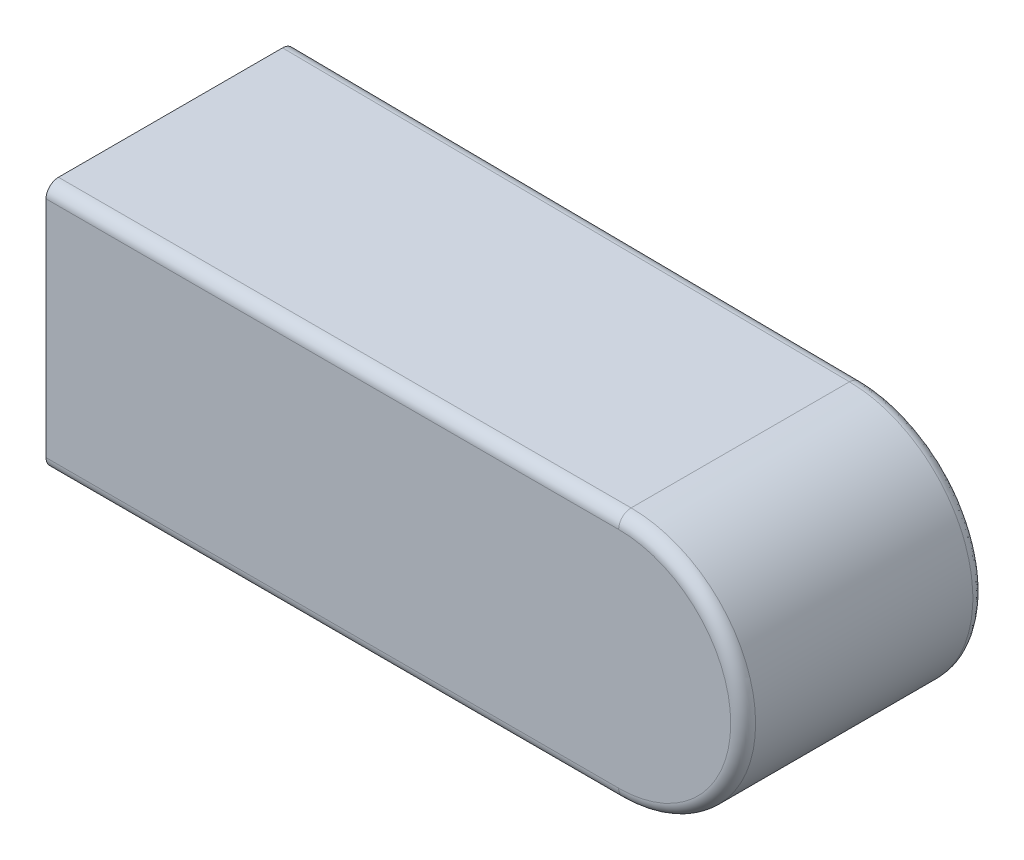
SolidWorks part; units mm, degrees
ref_plane "Front Plane" through (0, 0, 0) normal (0, 0, 1) x (1, 0, 0)
ref_plane "Top Plane" through (0, 0, 0) normal (0, 1, 0) x (1, 0, 0)
ref_plane "Right Plane" through (0, 0, 0) normal (1, 0, 0) x (0, 0, -1)
sketch "Dimension Sketch" plane through (0, 0, 0) normal (0, 1, 0) x (1, 0, 0)
  line L0 (0, 0) -> (14, 0) construction
  line L1 (0, 0) -> (0, 5) construction
  point P3 (5, 0)
  point P5 (5.25, 0)
  dimension "L" = 14
  dimension "b" = 5
  dimension "h" = 5
  dimension "r" = 0.25
sketch "Sketch1" plane through (0, 0, 0) normal (0, 0, 1) x (1, 0, 0)
  line L0 (-7, 2.5) -> (4.5, 2.5)
  line L1 (0, -1) -> (0, 1) construction
  line L2 (4.5, -2.5) -> (-7, -2.5)
  line L3 (-7, 0) -> (7, 0) construction
  line L4 (-7, 2.5) -> (-7, -2.5)
  arc A1 (4.5, 2.5) -> (4.5, -2.5) centre (4.5, 0) cw
  dimension "lm" = 14
  dimension "b" = 5
extrude "Extrude1" add sketch "Sketch1" along normal blind 5
sketch "Sketch2" plane through (0, 0, 0) normal (0, 1, 0) x (1, 0, 0)
  line L0 (7, -5) -> (107, -5) construction
  line L1 (7, -5) -> (7, 0) construction
  line L3 (7, -5) -> (7, -4) construction
  line L4 (-7, 0) -> (7, 0)
  line L5 (7, 0) -> (7, -0.14)
  line L6 (-7, 0) -> (7, -0.14)
  line L7 (7, -5) -> (7, 0) construction
  line L8 (7, -4) -> (107, -5) construction
  dimension "D1" = 100
  dimension "D2" = 1
extrude "Cut-Extrude1" cut sketch "Sketch2" against normal through all and the other way through all
fillet "Fillet2" radius 0.25 6 edges at (7, 0, 5) (-1.25, -2.5, 5) (-1.25, 2.5, 5) (-1.25, 2.5, 0.0575) (7, 0, 0.14) (-1.25, -2.5, 0.0575)
